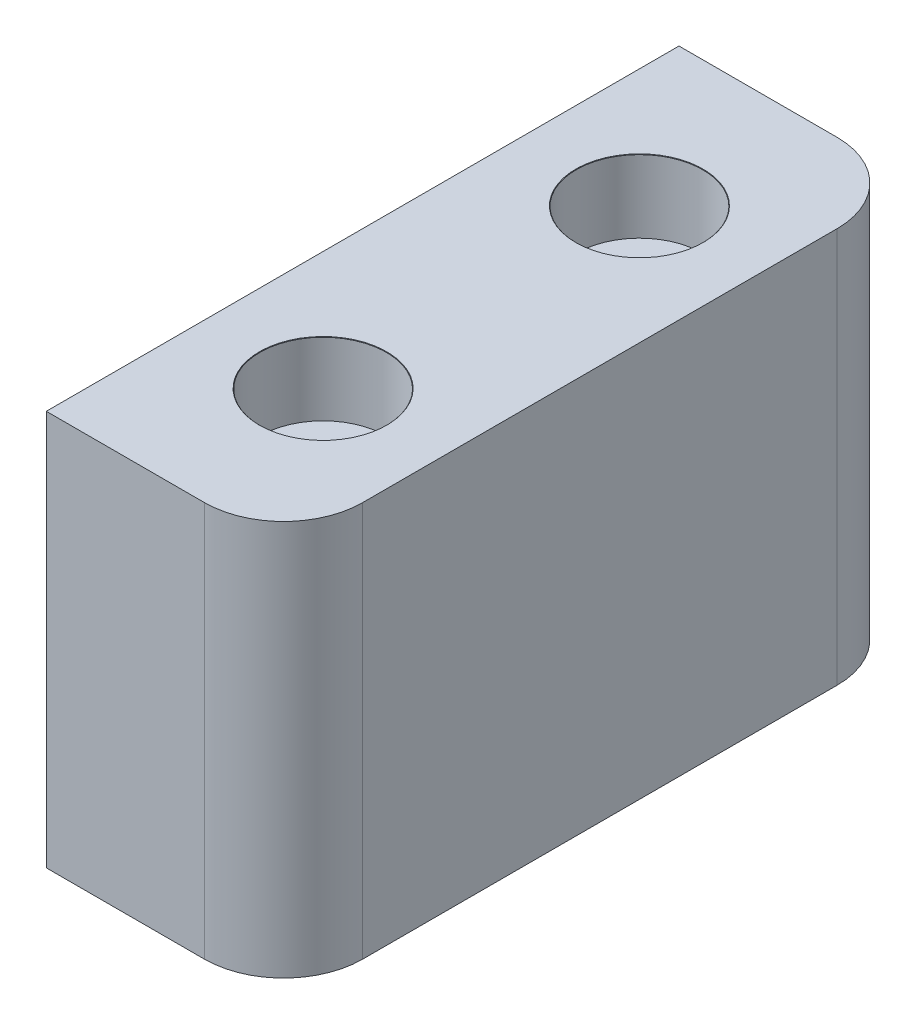
SolidWorks part; units mm, degrees
ref_plane "Front Plane" through (0, 0, 0) normal (0, 0, 1) x (1, 0, 0)
ref_plane "Top Plane" through (0, 0, 0) normal (0, 1, 0) x (1, 0, 0)
ref_plane "Right Plane" through (0, 0, 0) normal (1, 0, 0) x (0, 0, -1)
sketch "Sketch1" plane through (0, 0, 0) normal (0, 1, 0) x (1, 0, 0)
  line L1 (-7.5, -20) -> (7.5, -20)
  line L2 (-7.5, -20) -> (-7.5, 20)
  line L3 (-7.5, 20) -> (7.5, 20)
  line L4 (7.5, -20) -> (7.5, 20)
  line L5 (-7.5, -20) -> (7.5, 20) construction
  line L6 (-7.5, 20) -> (7.5, -20) construction
  point P0 (0, 0)
  dimension "D1" = 40
  dimension "D2" = 15
extrude "Boss-Extrude1" add sketch "Sketch1" along normal blind 25
fillet "Fillet1" radius 5 2 edges at (7.5, 12.5, 20) (7.5, 12.5, -20)
hole_wizard "Hole wizard: socket head cap screw, type 1" positions "Sketch2" profile "Sketch3" counterbore size "M4" standard "GB" end condition through all
sketch "Sketch2" plane through (0, 25, 0) normal (0, 1, 0) x (1, 0, 0)
  line L1 (0, 0) -> (50000, 0) construction
  line L2 (7.5, -15) -> (7.5, 15) construction
  point P0 (0, 10)
  point P11 (7.5, 0)
  point P13 (0, -10)
  dimension "D1" = 10
sketch "Sketch3" plane through (0, 25, -10) normal (1, 0, 0) x (0, 0, 1)
  line L0 (0, 0) -> (0, 25)
  line L1 (0, 25) -> (2.25, 25)
  line L3 (2.25, 25) -> (2.25, 4.6)
  line L4 (4, 4.6) -> (2.25, 4.6)
  line L5 (4, 4.6) -> (4, 0.025)
  line L6 (4, 0.025) -> (4.025, 0)
  line L7 (4.025, 0) -> (0, 0)
  line L8 (-4, 0.025) -> (-4.025, 0) construction
  line L11 (0, -6.35) -> (0, 107.95) construction
  dimension "通孔孔直径" = 4.5
  dimension "通孔孔深度" = 25
  dimension "柱形沉头孔直径" = 8
  dimension "柱形沉头孔深度" = 4.6
  dimension "近端锥形沉头孔直径" = 8.05
  dimension "近端锥形沉头孔角度" = 90
